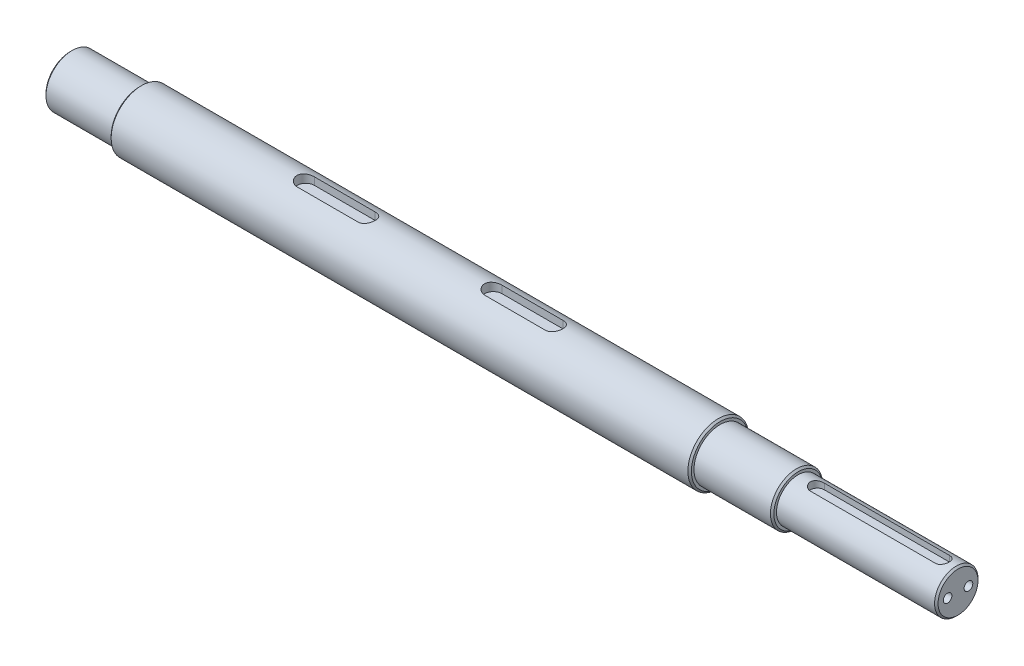
from build123d import *

# Parameters (mm, degrees)
CUT_EXTRUDE_1_DEPTH    = 5
CUT_EXTRUDE_2_DEPTH    = 4
CHAMFER_1_SIZE         = 1
HOLE_WIZARD_M6_1_D     = 5
HOLE_WIZARD_M6_1_DEPTH = 20
HOLE_WIZARD_M6_1_TIP   = 1.502151548


with BuildPart() as part:
    # 草图1 → 旋转1 (revolve)
    with BuildSketch(Plane.XY, mode=Mode.PRIVATE) as revolve_1_sk:
        Polygon((167, 17.5), (0, 17.5), (-167, 17.5), (-167, 15), (-207, 15), (-207, 0), (304, 0), (304, 12.5), (212, 12.5), (212, 15), (167, 15), align=None)
    revolve(revolve_1_sk.sketch.rotate(Axis((0, 0, 0), (-1, 0, 0)), 90), axis=Axis((0, 0, 0), (-1, 0, 0)))

    # 草图2 → 切除-拉伸1 (cut)
    with BuildSketch(Plane(origin=(0, 17.5, 0), x_dir=(1, 0, 0), z_dir=(0, 1, 0))):
        with BuildLine():
            Line((36.5, 5), (71.5, 5))
            ThreePointArc((71.5, 5), (76.5, 0), (71.5, -5))
            Line((71.5, -5), (36.5, -5))
            ThreePointArc((36.5, -5), (31.5, 0), (36.5, 5))
        make_face()
        with BuildLine():
            Line((-36.5, 5), (-71.5, 5))
            ThreePointArc((-71.5, 5), (-76.5, 0), (-71.5, -5))
            Line((-71.5, -5), (-36.5, -5))
            ThreePointArc((-36.5, -5), (-31.5, 0), (-36.5, 5))
        make_face()
    extrude(amount=-CUT_EXTRUDE_1_DEPTH, mode=Mode.SUBTRACT)

    # 草图3 → 切除-拉伸2 (cut)
    with BuildSketch(Plane(origin=(0, 12.5, 0), x_dir=(1, 0, 0), z_dir=(0, 1, 0))):
        with BuildLine():
            Line((223, 4), (295, 4))
            ThreePointArc((295, 4), (299, 0), (295, -4))
            Line((295, -4), (223, -4))
            ThreePointArc((223, -4), (219, 0), (223, 4))
        make_face()
    extrude(amount=-CUT_EXTRUDE_2_DEPTH, mode=Mode.SUBTRACT)

    # 倒角1
    chamfer_1_edges = [part.edges().sort_by_distance(p)[0] for p in [
        (-207, 0, 15),
        (-167, 0, 17.5),
        (167, 0, 17.5),
        (212, 0, 15),
        (304, 0, 12.5),
    ]]
    chamfer(chamfer_1_edges, length=CHAMFER_1_SIZE)

    # M6 螺纹孔1
    with Locations(Plane(origin=(304, 0, 0), x_dir=(0, 0, -1), z_dir=(1, 0, 0))):
        with Locations((6, 0), (-6, 0)):
            Hole(HOLE_WIZARD_M6_1_D / 2, depth=HOLE_WIZARD_M6_1_DEPTH)
            with Locations((0, 0, -(HOLE_WIZARD_M6_1_DEPTH + HOLE_WIZARD_M6_1_TIP / 2))):  # 118° drill point
                Cone(0, HOLE_WIZARD_M6_1_D / 2, HOLE_WIZARD_M6_1_TIP, mode=Mode.SUBTRACT)


solid = part.part
